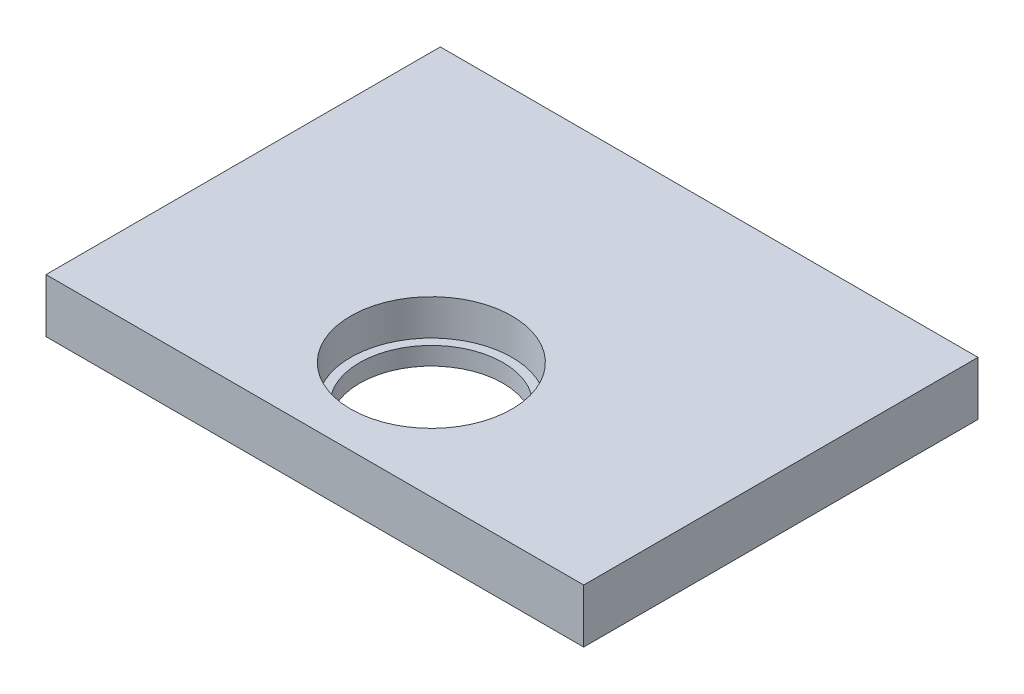
from build123d import *

# Parameters (mm, degrees)
SKETCH_1_W          = 300
SKETCH_1_H          = 220
EXTRUDE_1_DEPTH     = 30
SKETCH_2_R          = 45
CUT_EXTRUDE_1_DEPTH = 20
SKETCH_3_R          = 40
CUT_EXTRUDE_2_DEPTH = 189.414436814


with BuildPart() as part:
    # 草图1 → 凸台-拉伸1 (new body)
    with BuildSketch(Plane(origin=(0, 0, 0), x_dir=(1, 0, 0), z_dir=(0, 1, 0))):
        Rectangle(SKETCH_1_W, SKETCH_1_H)
    extrude(amount=EXTRUDE_1_DEPTH)

    # 草图2 → 切除-拉伸1 (cut)
    with BuildSketch(Plane(origin=(0, 30, 0), x_dir=(1, 0, 0), z_dir=(0, 1, 0))):
        with Locations(Location((0, -45, 0), (0, 0, 270))):
            Circle(SKETCH_2_R)
    extrude(amount=-CUT_EXTRUDE_1_DEPTH, mode=Mode.SUBTRACT)

    # 草图3 → 切除-拉伸2 (cut, through all)
    with BuildSketch(Plane(origin=(0, 30, 0), x_dir=(1, 0, 0), z_dir=(0, 1, 0))):
        with Locations(Location((0, -45, 0), (0, 0, 270))):
            Circle(SKETCH_3_R)
    extrude(amount=-CUT_EXTRUDE_2_DEPTH, mode=Mode.SUBTRACT)


solid = part.part
